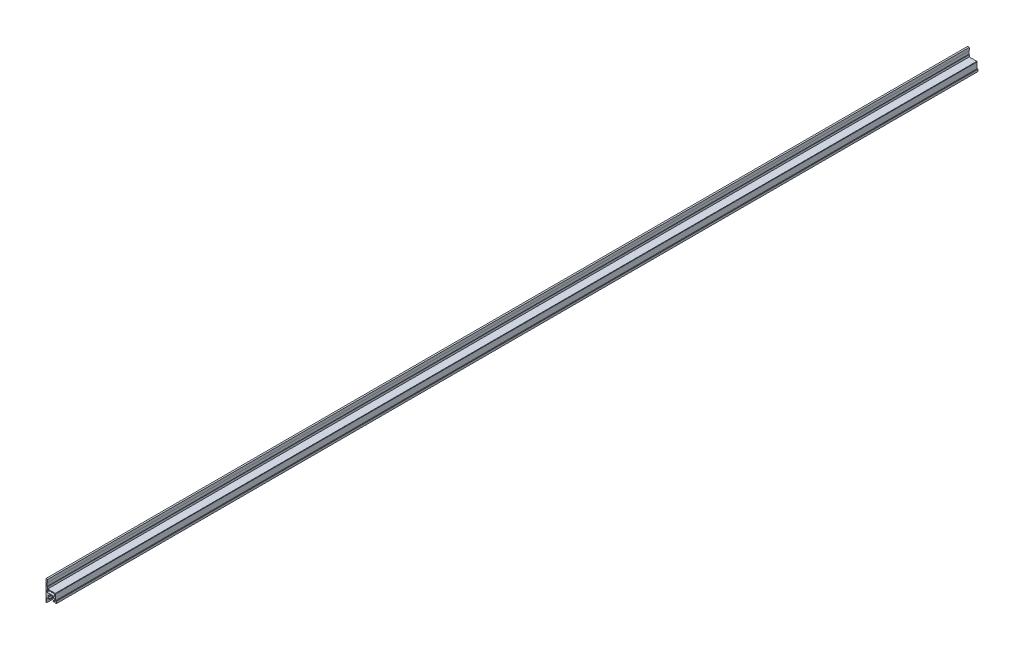
from build123d import *

# Parameters (mm, degrees)
SKETCH_2_W      = 19
SKETCH_2_H      = 5.6
EXTRUDE_1_DEPTH = 1108


with BuildPart() as part:
    # 草图2 → 凸台-拉伸1 (new, symmetric)
    with BuildSketch(Plane.XY):
        with BuildLine():
            Line((1.5, 10), (4, 10))
            Line((4, 10), (4, 10.5))
            Line((4, 10.5), (8.9, 10.5))
            Line((8.9, 10.5), (8.9, 12.2))
            ThreePointArc((8.9, 12.2), (8.812132034, 12.412132034), (8.6, 12.5))
            Line((8.6, 12.5), (5.05, 12.5))
            ThreePointArc((5.05, 12.5), (4.837867966, 12.587867966), (4.75, 12.8))
            Line((4.75, 12.8), (4.75, 16.152943725))
            ThreePointArc((4.75, 16.152943725), (4.77283614, 16.267748755), (4.837867966, 16.36507576))
            Line((4.837867966, 16.36507576), (8.78492424, 20.312132034))
            ThreePointArc((8.78492424, 20.312132034), (8.882251245, 20.37716386), (8.997056275, 20.4))
            Line((8.997056275, 20.4), (17.002943725, 20.4))
            ThreePointArc((17.002943725, 20.4), (17.117748755, 20.37716386), (17.21507576, 20.312132034))
            Line((17.21507576, 20.312132034), (21.162132034, 16.36507576))
            ThreePointArc((21.162132034, 16.36507576), (21.22716386, 16.267748755), (21.25, 16.152943725))
            Line((21.25, 16.152943725), (21.25, 12.8))
            ThreePointArc((21.25, 12.8), (21.162132034, 12.587867966), (20.95, 12.5))
            Line((20.95, 12.5), (17.4, 12.5))
            ThreePointArc((17.4, 12.5), (17.187867966, 12.412132034), (17.1, 12.2))
            Line((17.1, 12.2), (17.1, 10.5))
            Line((17.1, 10.5), (22, 10.5))
            Line((22, 10.5), (22, 10))
            Line((22, 10), (25, 10))
            Line((25, 10), (25, 15))
            Line((25, 15), (23, 15))
            Line((23, 15), (23, 29.24572809))
            Line((23, 29.24572809), (22.25, 29.99572809))
            Line((22.25, 29.99572809), (4, 30))
            Line((4, 30), (4, 34.998393128))
            Line((4, 34.998393128), (3, 34.998393128))
            Line((3, 34.998393128), (3, 43))
            Line((3, 43), (4, 43))
            Line((4, 43), (4, 50))
            Line((4, 50), (0, 50))
            Line((0, 50), (0, 0))
            Line((0, 0), (1.5, 0))
            Line((1.5, 0), (1.5, 10))
        make_face()
        with Locations((11.5, 25.2)):
            Rectangle(SKETCH_2_W, SKETCH_2_H, mode=Mode.SUBTRACT)
    extrude(amount=EXTRUDE_1_DEPTH, both=True)


solid = part.part
